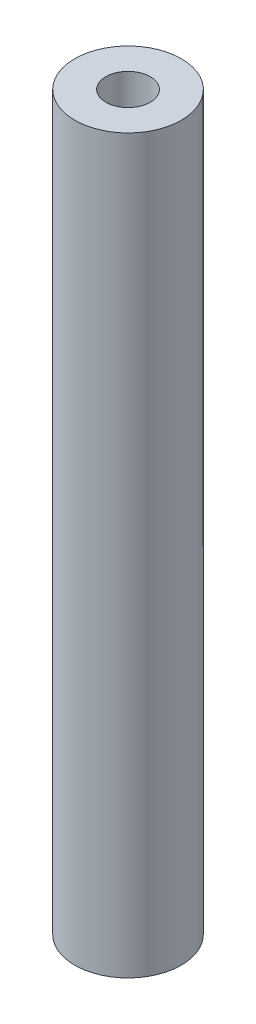
from build123d import *

# Parameters (mm, degrees)
SKETCH_1_R         = 3
EXTRUDE_1_DEPTH    = 41.2
HOLE_WIZARD_M3_1_D = 2.5


with BuildPart() as part:
    # 草图1 → 凸台-拉伸1 (new body)
    with BuildSketch(Plane(origin=(0, 0, 0), x_dir=(1, 0, 0), z_dir=(0, 1, 0))):
        with Locations(Location((0, 0, 0), (0, 0, 90))):
            Circle(SKETCH_1_R)
    extrude(amount=EXTRUDE_1_DEPTH)

    # M3 螺纹孔1 (through all)
    with Locations(Plane(origin=(0, 41.2, 0), x_dir=(1, 0, 0), z_dir=(0, 1, 0))):
        with Locations((0, 0)):
            Hole(HOLE_WIZARD_M3_1_D / 2)


solid = part.part
